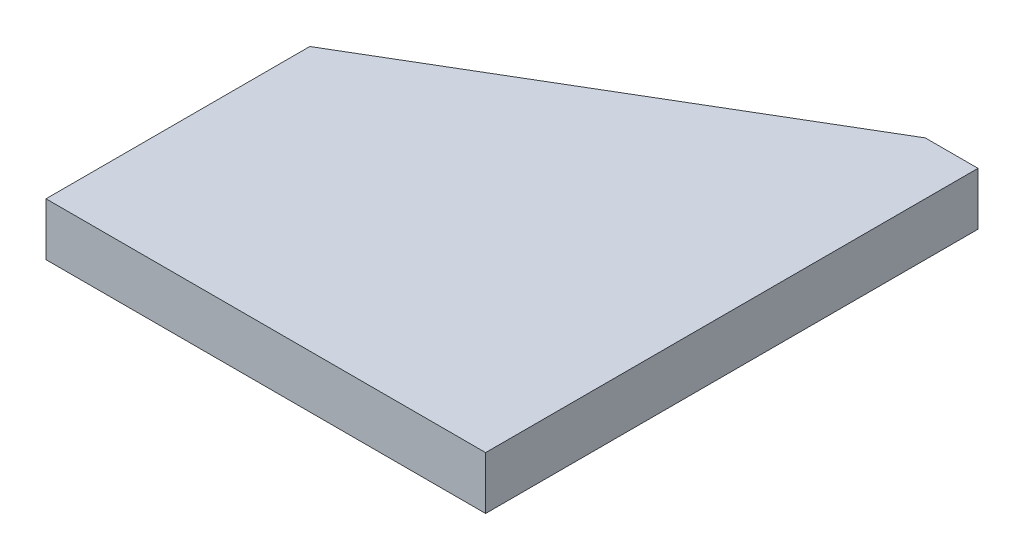
SolidWorks part; units mm, degrees
ref_plane "前视基准面" through (0, 0, 0) normal (0, 0, 1) x (1, 0, 0)
ref_plane "上视基准面" through (0, 0, 0) normal (0, 1, 0) x (1, 0, 0)
ref_plane "右视基准面" through (0, 0, 0) normal (1, 0, 0) x (0, 0, -1)
sketch "草图1" plane through (0, 0, 0) normal (0, 1, 0) x (1, 0, 0)
  line L0 (162.7907, 182.3256) -> (132.7907, 182.3256)
  line L1 (-87.2093, -97.6744) -> (162.7907, -97.6744)
  line L2 (-87.2093, -97.6744) -> (-87.2093, 52.3256)
  line L4 (162.7907, -97.6744) -> (162.7907, 182.3256)
  line L5 (-87.2093, -97.6744) -> (162.7907, 182.3256) construction
  line L6 (-87.2093, 52.3256) -> (162.7907, -97.6744) construction
  line L7 (132.7907, 182.3256) -> (-87.2093, 52.3256)
  point P0 (0, 0)
  dimension "D1" = 150
  dimension "D2" = 250
  dimension "D3" = 280
  dimension "D4" = 30
extrude "凸台-拉伸1" add sketch "草图1" along normal blind 30
